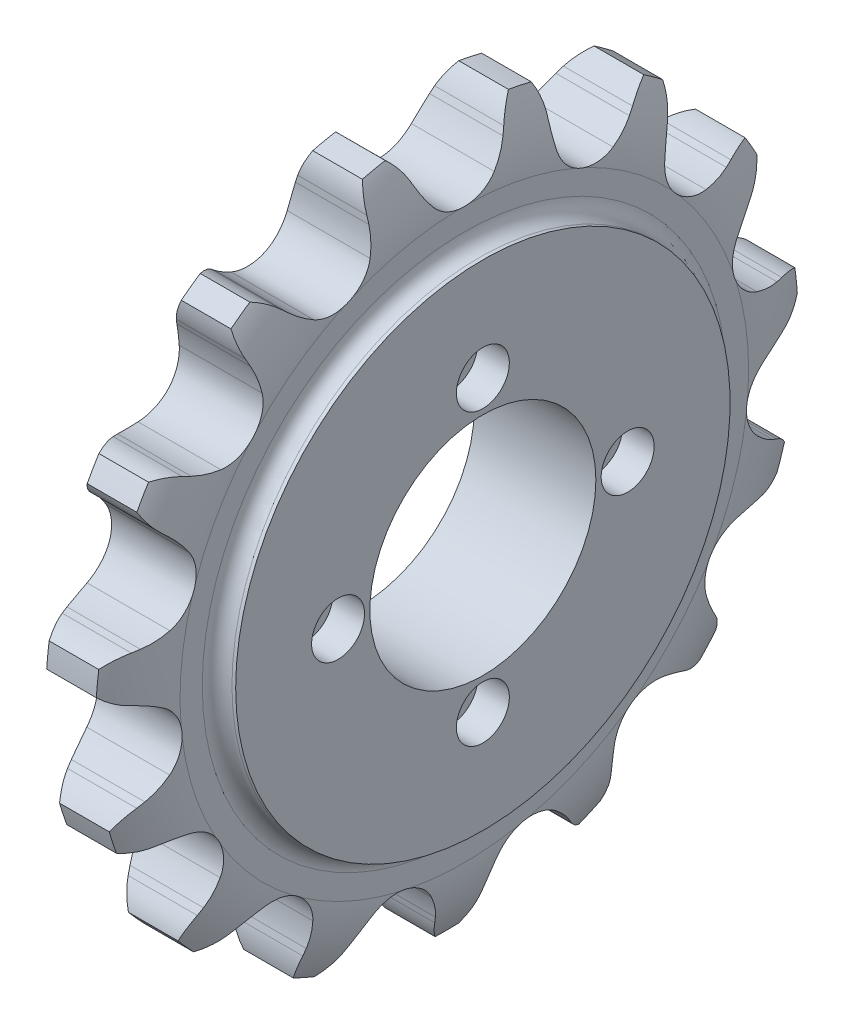
from build123d import *

# Parameters (mm, degrees)
EXTRUDECUTONE_DEPTH       = 16.984719634
PATTERNONE_COUNT          = 15
CUT_EXTRUDEA_DEPTH        = 142.587656458
CUT_EXTRUDEA_DEPTH_BACK   = 142.587656458
SKETCHHOLE_R              = 10
CUT_EXTRUDEB_DEPTH        = 142.587656458
CUT_EXTRUDEB_DEPTH_BACK   = 142.587656458
SKETCHKEY_W               = 6
SKETCHKEY_H               = 7.799999952
HOLE_WIZARD_1_D           = 9
HOLE_WIZARD_1_CBORE_D     = 15
HOLE_WIZARD_1_CBORE_DEPTH = 9
SKETCH_5_R                = 32
CUT_EXTRUDE_3_DEPTH       = 145.700280386


with BuildPart() as part:
    # Sketch1 → Revolve 2 (revolve)
    with BuildSketch(Plane.XY, mode=Mode.PRIVATE) as revolve_2_sk:
        with BuildLine():
            Line((-17.234719634, 0), (-17.234719634, 70))
            Line((-17.234719634, 70), (-16.183675707, 70))
            ThreePointArc((-16.183675707, 70), (-13.210874555, 71.231374555), (-11.9795, 74.204175707))
            Line((-11.9795, 74.204175707), (-11.9795, 80.510439267))
            ThreePointArc((-11.9795, 80.510439267), (-10.746639243, 90.329594971), (-7.0265, 99.5))
            Line((-7.0265, 99.5), (7.0265, 99.5))
            ThreePointArc((7.0265, 99.5), (10.746639243, 90.329594971), (11.9795, 80.510439267))
            Line((11.9795, 80.510439267), (11.9795, 74.204175707))
            ThreePointArc((11.9795, 74.204175707), (13.210874555, 71.231374555), (16.183675707, 70))
            Line((16.183675707, 70), (17.234719634, 70))
            Line((17.234719634, 70), (17.234719634, 0))
            Line((17.234719634, 0), (-17.234719634, 0))
        make_face()
    revolve(revolve_2_sk.sketch.rotate(Axis((-4, 0, 0), (1, 0, 0)), 90), axis=Axis((-4, 0, 0), (1, 0, 0)))

    # Sketch2 → ExtrudeCutOne (cut, symmetric)
    with BuildSketch(Plane(origin=(0, 0, 0), x_dir=(0, 0, -1), z_dir=(1, 0, 0))):
        with BuildLine():
            Line((12.523074172, 90.681887943), (13.354481298, 92.486730089))
            ThreePointArc((13.354481298, 92.486730089), (15.10924996, 95.437983979), (17.439423475, 97.959769849))
            ThreePointArc((17.439423475, 97.959769849), (0, 99.5), (-17.439423475, 97.959769849))
            ThreePointArc((-17.439423475, 97.959769849), (-15.10924996, 95.437983979), (-13.354481298, 92.486730089))
            Line((-13.354481298, 92.486730089), (-12.523074172, 90.681887943))
            ThreePointArc((-12.523074172, 90.681887943), (-10.812212003, 87.504472082), (-8.720024546, 84.564102621))
            ThreePointArc((-8.720024546, 84.564102621), (0, 80.404864267), (8.720024546, 84.564102621))
            ThreePointArc((8.720024546, 84.564102621), (10.812212003, 87.504472082), (12.523074172, 90.681887943))
        make_face()
    extrudecutone = extrude(amount=EXTRUDECUTONE_DEPTH, both=True, mode=Mode.SUBTRACT)

    # PatternOne: ExtrudeCutOne ×15 about axis
    patternone_axis = Axis((0, 0, 0), (1, 0, 0))
    for i in range(1, PATTERNONE_COUNT):
        add(extrudecutone.rotate(patternone_axis, i * 360 / PATTERNONE_COUNT), mode=Mode.SUBTRACT)

    # SketchHole → Cut-ExtrudeA (cut, two sides: drawn at the far end of the back side and taken through both)
    with BuildSketch(Plane(origin=(0, 0, 0), x_dir=(0, 0, -1), z_dir=(1, 0, 0)).offset(-CUT_EXTRUDEA_DEPTH_BACK)):
        Circle(SKETCHHOLE_R)
    extrude(amount=CUT_EXTRUDEA_DEPTH + CUT_EXTRUDEA_DEPTH_BACK, mode=Mode.SUBTRACT)

    # SketchKey → Cut-ExtrudeB (cut, two sides: drawn at the far end of the back side and taken through both)
    with BuildSketch(Plane(origin=(0, 0, 0), x_dir=(0, 0, -1), z_dir=(1, 0, 0)).offset(-CUT_EXTRUDEB_DEPTH_BACK)):
        with Locations((0, 8.899999976)):
            Rectangle(SKETCHKEY_W, SKETCHKEY_H)
    extrude(amount=CUT_EXTRUDEB_DEPTH + CUT_EXTRUDEB_DEPTH_BACK, mode=Mode.SUBTRACT)

    # 打孔尺寸(%根据)内六角圆柱头螺钉的类型1 (through all)
    with Locations(Plane(origin=(17.234719634, 0, 0), x_dir=(0, 0, -1), z_dir=(1, 0, 0))):
        with Locations((0, 41), (41, 0), (0, -41), (-41, 0)):
            CounterBoreHole(HOLE_WIZARD_1_D / 2, HOLE_WIZARD_1_CBORE_D / 2, HOLE_WIZARD_1_CBORE_DEPTH)

    # 草图5 → 切除-拉伸3 (cut, through all)
    with BuildSketch(Plane(origin=(17.234719634, 0, 0), x_dir=(0, 0, -1), z_dir=(1, 0, 0))):
        Circle(SKETCH_5_R)
    extrude(amount=-CUT_EXTRUDE_3_DEPTH, mode=Mode.SUBTRACT)


solid = part.part
